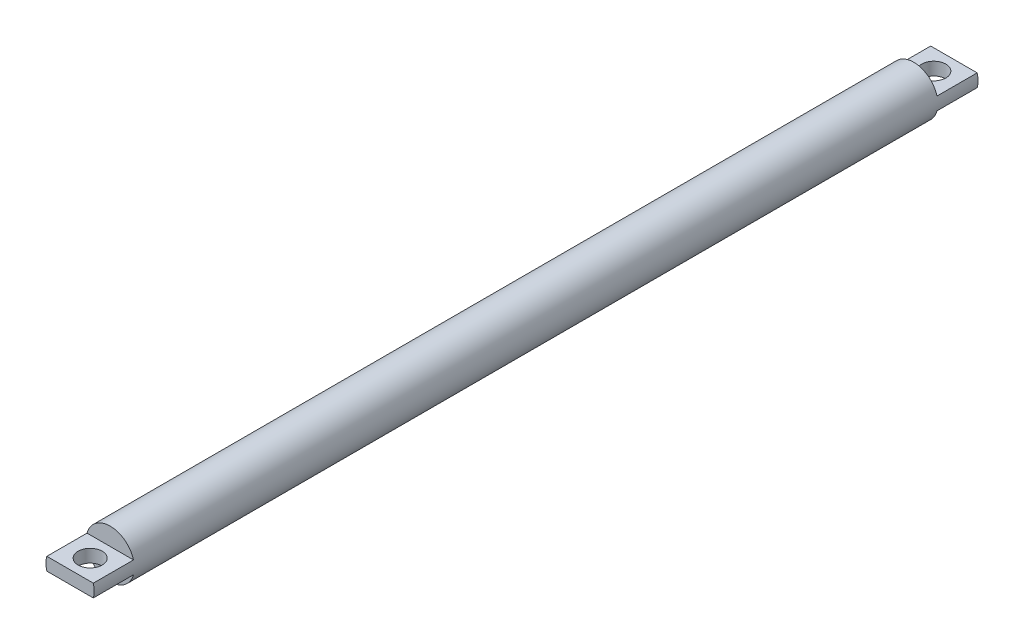
from build123d import *
from build123d.topology import SkipClean

# Parameters (mm, degrees)
SKETCH_1_R          = 3
EXTRUDE_1_DEPTH     = 100
EXTRUDE_3_DEPTH     = 5
EXTRUDE_START       = 5
EXTRUDE_4_DEPTH     = 5
SKETCH_9_R          = 1.5
CUT_EXTRUDE_1_DEPTH = 5
SKETCH_10_R         = 1.5
CUT_EXTRUDE_2_DEPTH = 5


with BuildPart() as part:
    # 草图1 → 凸台-拉伸1 (new body)
    with BuildSketch(Plane.XY):
        Circle(SKETCH_1_R)
    extrude(amount=EXTRUDE_1_DEPTH)

    # 草图2 → 凸台-拉伸3 (add)
    with SkipClean():  # the faces are left unmerged after this step: merging them gives an invalid solid
        with BuildSketch(Plane.XY.offset(100)):
            with BuildLine():
                Line((-2.891366459, 0.8), (2.891366459, 0.8))
                ThreePointArc((2.891366459, 0.8), (3, 0), (2.891366459, -0.8))
                Line((2.891366459, -0.8), (-2.891366459, -0.8))
                ThreePointArc((-2.891366459, -0.8), (-3, 0), (-2.891366459, 0.8))
            make_face()
        extrude(amount=EXTRUDE_3_DEPTH)

    # 草图8 → 凸台-拉伸4 (add)
    with SkipClean():  # the faces are left unmerged after this step: merging them gives an invalid solid
        with BuildSketch(Plane(origin=(0, 0, 0), x_dir=(-1, 0, 0), z_dir=(0, 0, -1)).offset(EXTRUDE_START)):
            with BuildLine():
                Line((-2.891366459, 0.8), (2.891366459, 0.8))
                ThreePointArc((2.891366459, 0.8), (3, 0), (2.891366459, -0.8))
                Line((2.891366459, -0.8), (-2.891366459, -0.8))
                ThreePointArc((-2.891366459, -0.8), (-3, 0), (-2.891366459, 0.8))
            make_face()
        extrude(amount=-EXTRUDE_4_DEPTH)

    # 草图9 → 切除-拉伸1 (cut)
    with SkipClean():  # the faces are left unmerged after this step: merging them gives an invalid solid
        with BuildSketch(Plane(origin=(0, 0.8, 0), x_dir=(1, 0, 0), z_dir=(0, 1, 0))):
            with Locations(Location((0, 2.5, 0), (0, 0, 270))):
                Circle(SKETCH_9_R)
        extrude(amount=-CUT_EXTRUDE_1_DEPTH, mode=Mode.SUBTRACT)

    # 草图10 → 切除-拉伸2 (cut)
    with SkipClean():  # the faces are left unmerged after this step: merging them gives an invalid solid
        with BuildSketch(Plane(origin=(0, 0.8, 0), x_dir=(1, 0, 0), z_dir=(0, 1, 0))):
            with Locations(Location((0, -102.5, 0), (0, 0, 270))):
                Circle(SKETCH_10_R)
        extrude(amount=-CUT_EXTRUDE_2_DEPTH, mode=Mode.SUBTRACT)


solid = part.part
